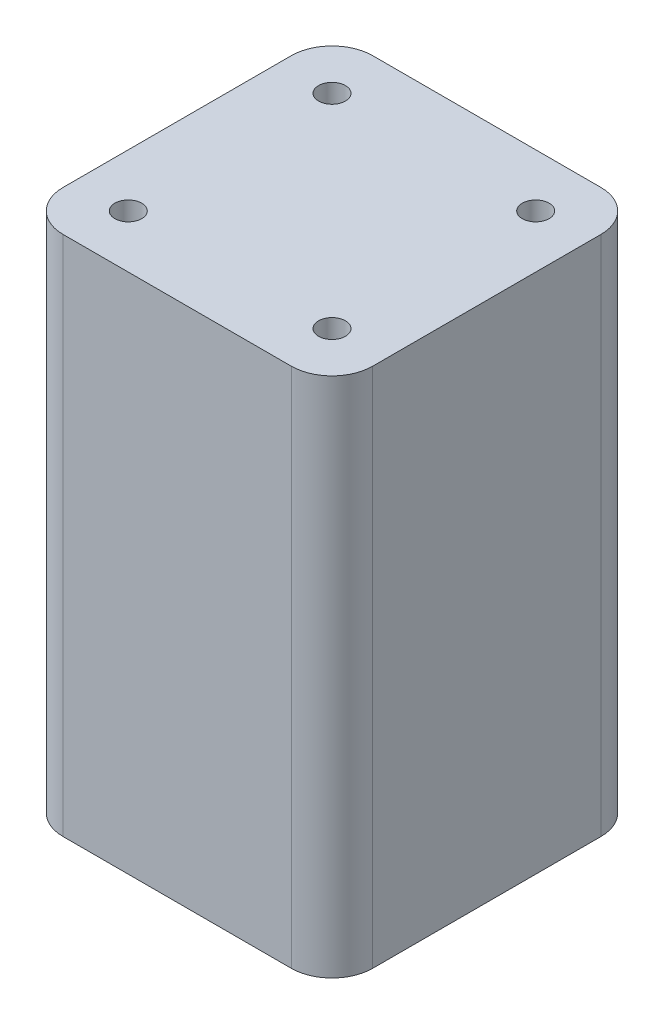
from build123d import *

# Parameters (mm, degrees)
SKETCH1_W             = 38
SKETCH1_H             = 68
BOSS_EXTRUDE1_DEPTH   = 10
SKETCH2_W             = 38
SKETCH2_H             = 38
BOSS_EXTRUDE2_DEPTH   = 54
M4_TAPPED_HOLE2_D     = 3.3
M4_TAPPED_HOLE2_DEPTH = 10.1
M4_TAPPED_HOLE2_TIP   = 0.99142
FILLET1_R             = 5
M4_TAPPED_HOLE1_D     = 3.3
M4_TAPPED_HOLE1_DEPTH = 10.1
M4_TAPPED_HOLE1_TIP   = 0.99142
SKETCH8_OUTSIDE_W     = 60.164
SKETCH8_OUTSIDE_H     = 90.164
CUT_EXTRUDE1_DEPTH    = 75.919957


with BuildPart() as part:
    # Sketch1 → Boss-Extrude1 (new body)
    with BuildSketch(Plane(origin=(0, 0, 0), x_dir=(1, 0, 0), z_dir=(0, 1, 0))):
        Rectangle(SKETCH1_W, SKETCH1_H)
    extrude(amount=BOSS_EXTRUDE1_DEPTH)

    # Sketch2 → Boss-Extrude2 (add)
    with BuildSketch(Plane(origin=(0, 10, 0), x_dir=(1, 0, 0), z_dir=(0, 1, 0))):
        Rectangle(SKETCH2_W, SKETCH2_H)
    extrude(amount=BOSS_EXTRUDE2_DEPTH)

    # M4 Tapped Hole2
    with Locations(Plane.XZ):
        with Locations((-12.5, -12.5), (12.5, -12.5), (-12.5, 12.5), (12.5, 12.5)):
            Hole(M4_TAPPED_HOLE2_D / 2, depth=M4_TAPPED_HOLE2_DEPTH)
            with Locations((0, 0, -(M4_TAPPED_HOLE2_DEPTH + M4_TAPPED_HOLE2_TIP / 2))):  # 118° drill point
                Cone(0, M4_TAPPED_HOLE2_D / 2, M4_TAPPED_HOLE2_TIP, mode=Mode.SUBTRACT)

    # Fillet1
    fillet1_edges = [part.edges().sort_by_distance(p)[0] for p in [
        (19, 37, 19),
        (19, 37, -19),
        (-19, 37, -19),
        (-19, 37, 19),
        (19, 5, 34),
        (-19, 5, 34),
        (-19, 5, -34),
        (19, 5, -34),
    ]]
    fillet(fillet1_edges, radius=FILLET1_R)

    # M4 Tapped Hole1
    with Locations(Plane(origin=(0, 64, 0), x_dir=(1, 0, 0), z_dir=(0, 1, 0))):
        with Locations((-12.5, 12.5), (12.5, 12.5), (12.5, -12.5), (-12.5, -12.5)):
            Hole(M4_TAPPED_HOLE1_D / 2, depth=M4_TAPPED_HOLE1_DEPTH)
            with Locations((0, 0, -(M4_TAPPED_HOLE1_DEPTH + M4_TAPPED_HOLE1_TIP / 2))):  # 118° drill point
                Cone(0, M4_TAPPED_HOLE1_D / 2, M4_TAPPED_HOLE1_TIP, mode=Mode.SUBTRACT)

    # Sketch8 outside → Cut-Extrude1 (cut, through all)
    with BuildSketch(Plane(origin=(0, 64, 0), x_dir=(1, 0, 0), z_dir=(0, 1, 0))):
        Rectangle(SKETCH8_OUTSIDE_W, SKETCH8_OUTSIDE_H)
        with BuildLine():
            Line((-14, 19), (14, 19))
            ThreePointArc((14, 19), (17.535534, 17.535534), (19, 14))
            Line((19, 14), (19, -14))
            ThreePointArc((19, -14), (17.535534, -17.535534), (14, -19))
            Line((14, -19), (-14, -19))
            ThreePointArc((-14, -19), (-17.535534, -17.535534), (-19, -14))
            Line((-19, -14), (-19, 14))
            ThreePointArc((-19, 14), (-17.535534, 17.535534), (-14, 19))
        make_face(mode=Mode.SUBTRACT)
    extrude(amount=-CUT_EXTRUDE1_DEPTH, mode=Mode.SUBTRACT)


solid = part.part
